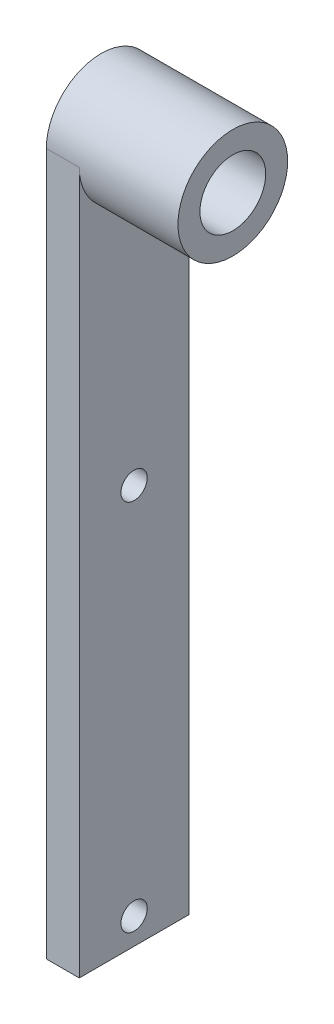
from build123d import *

# Parameters (mm, degrees)
SKETCH_1_W              = 50
SKETCH_1_H              = 320
EXTRUDE_1_DEPTH         = 7.5
EXTRUDE_2_DEPTH         = 52.5
EXTRUDE_2_DEPTH_BACK    = 7.5
SKETCH_2_R              = 25
SKETCH_3_R              = 15
CUT_EXTRUDE_1_DEPTH     = 197.086715511
HOLE_WIZARD_12_0_12_1_D = 12


with BuildPart() as part:
    # 草图1 → 凸台-拉伸1 (new, symmetric)
    with BuildSketch(Plane(origin=(0, 0, 0), x_dir=(0, 0, -1), z_dir=(1, 0, 0))):
        Rectangle(SKETCH_1_W, SKETCH_1_H)
    extrude(amount=EXTRUDE_1_DEPTH, both=True)

    # 草图2 → 凸台-拉伸2 (add, two sides: drawn at the far end of the back side and taken through both)
    with BuildSketch(Plane(origin=(0, 0, 0), x_dir=(0, 0, -1), z_dir=(1, 0, 0)).offset(-EXTRUDE_2_DEPTH_BACK)):
        with Locations((0, 160)):
            Circle(SKETCH_2_R)
    extrude(amount=EXTRUDE_2_DEPTH + EXTRUDE_2_DEPTH_BACK)

    # 草图3 → 切除-拉伸1 (cut, through all)
    with BuildSketch(Plane(origin=(52.5, 0, 0), x_dir=(0, 0, -1), z_dir=(1, 0, 0))):
        with Locations((0, 160)):
            Circle(SKETCH_3_R)
    extrude(amount=-CUT_EXTRUDE_1_DEPTH, mode=Mode.SUBTRACT)

    # Ø12.0 (12) 直径孔1 (through all)
    with Locations(Plane.ZY.offset(7.5)):
        with Locations((0, 22), (0, -148)):
            Hole(HOLE_WIZARD_12_0_12_1_D / 2)


solid = part.part
